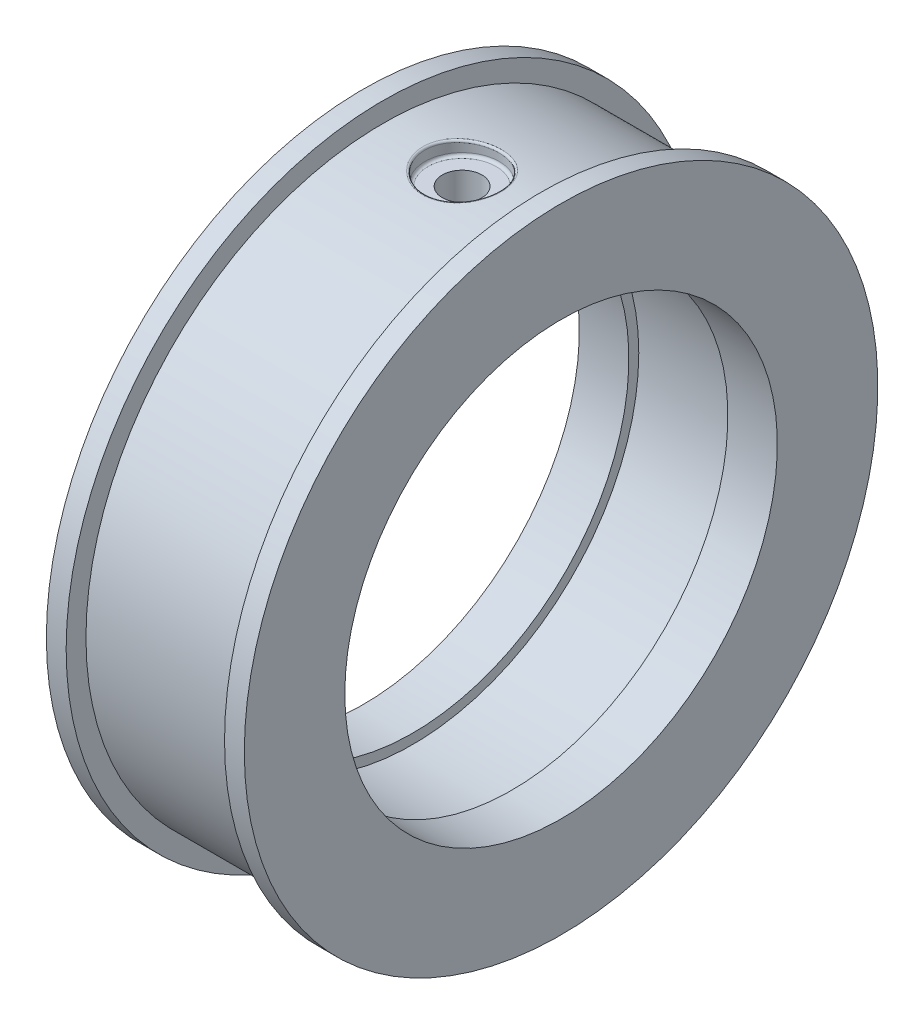
from build123d import *

# Parameters (mm, degrees)
HOLE1_D           = 7.5
HOLE1_DEPTH       = 1.5
HOLE2_REACH       = 71.419
HOLE2_BORE_R      = 2
DOWEL_HOLE1_D     = 4
DOWEL_HOLE1_DEPTH = 4
DOWEL_HOLE1_TIP   = 1.201721238
FILLET1_R         = 0.2
FILLET2_R         = 0.3


with BuildPart() as part:
    # Sketch1 → Revolve1 (revolve)
    with BuildSketch(Plane.XY, mode=Mode.PRIVATE) as revolve1_sk:
        Polygon((-8.389660143, 21.85), (-8.389660143, 32), (-6.389660143, 32), (-6.389660143, 30), (9.610339857, 30), (9.610339857, 32), (11.610339857, 32), (11.610339857, 21.85), (6.610339857, 21.85), (6.610339857, 22.85), (-3.389660143, 22.85), (-3.389660143, 21.85), align=None)
    revolve(revolve1_sk.sketch.rotate(Axis((-19.036826505, 0, 0), (1, 0, 0)), 90), axis=Axis((-19.036826505, 0, 0), (1, 0, 0)))

    # Hole1
    with Locations(Plane(origin=(0, 30, 0), x_dir=(1, 0, 0), z_dir=(0, 1, 0))):
        with Locations((1.610339857, 0)):
            Hole(HOLE1_D / 2, depth=HOLE1_DEPTH)

    # Hole2 bore → Hole2 (cut, up to next)
    with BuildSketch(Plane(origin=(0, 28.5, 0), x_dir=(1, 0, 0), z_dir=(0, 1, 0)), mode=Mode.PRIVATE) as hole2_sk1:
        with Locations((1.610339857, 0)):
            Circle(HOLE2_BORE_R)
    hole2_tool1 = extrude(hole2_sk1.sketch, amount=-HOLE2_REACH, mode=Mode.PRIVATE) & part.part
    add(hole2_tool1.solids().sort_by_distance((1.61034, 28.5, 0))[0], mode=Mode.SUBTRACT)

    # Dowel Hole1
    with Locations(Plane(origin=(0, -30, 0), x_dir=(-1, 0, 0), z_dir=(0, -1, 0))):
        with Locations((-1.610339857, 0)):
            Hole(DOWEL_HOLE1_D / 2, depth=DOWEL_HOLE1_DEPTH)
            with Locations((0, 0, -(DOWEL_HOLE1_DEPTH + DOWEL_HOLE1_TIP / 2))):  # 118° drill point
                Cone(0, DOWEL_HOLE1_D / 2, DOWEL_HOLE1_TIP, mode=Mode.SUBTRACT)

    # Fillet1
    fillet1_edges = [part.edges().sort_by_distance(p)[0] for p in [
        (5.360339864, 29.999999997, -1e-09),
    ]]
    fillet(fillet1_edges, radius=FILLET1_R)

    # Fillet2
    fillet2_edges = [part.edges().sort_by_distance(p)[0] for p in [
        (5.360339857, 28.5, 0),
    ]]
    fillet(fillet2_edges, radius=FILLET2_R)


solid = part.part
